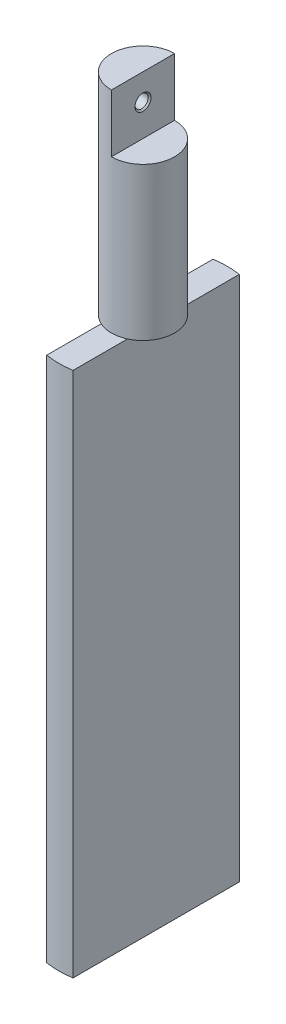
from build123d import *

# Parameters (mm, degrees)
SKETCH1_R                   = 6
BOSS_EXTRUDE1_DEPTH         = 40
CUT_EXTRUDE1_DEPTH          = 41.890096601
CUT_EXTRUDE1_DEPTH_BACK     = 41.890096601
SKETCH2_W                   = 18.470240229
SKETCH2_H                   = 11
M3_TAPPED_HOLE2_D           = 2.5
M3_TAPPED_HOLE2_CSINK_D     = 3.05
M3_TAPPED_HOLE2_CSINK_ANGLE = 90
SKETCH5_R                   = 16
BOSS_EXTRUDE2_DEPTH         = 100
CUT_EXTRUDE2_DEPTH          = 142.816783309
CUT_EXTRUDE2_DEPTH_BACK     = 100
SKETCH11_OUTSIDE_W          = 63.426
SKETCH11_OUTSIDE_H          = 63.426
SKETCH11_OUTSIDE_W_2        = 5
SKETCH11_OUTSIDE_H_2        = 40.425128238


with BuildPart() as part:
    # Sketch1 → Boss-Extrude1 (new body)
    with BuildSketch(Plane(origin=(0, 0, 0), x_dir=(1, 0, 0), z_dir=(0, 1, 0))):
        with Locations(Location((0, 0, 0), (0, 0, 270))):
            Circle(SKETCH1_R)
    extrude(amount=BOSS_EXTRUDE1_DEPTH)

    # Sketch2 → Cut-Extrude1 (cut, two sides: drawn at the far end of the back side and taken through both)
    with BuildSketch(Plane.XY.offset(-CUT_EXTRUDE1_DEPTH_BACK)):
        with Locations((9.235120115, 34.5)):
            Rectangle(SKETCH2_W, SKETCH2_H)
    extrude(amount=CUT_EXTRUDE1_DEPTH + CUT_EXTRUDE1_DEPTH_BACK, mode=Mode.SUBTRACT)

    # M3 Tapped Hole2 (through all)
    with Locations(Plane(origin=(0, 0, 0), x_dir=(0, 0, -1), z_dir=(1, 0, 0))):
        with Locations((0, 35)):
            CounterSinkHole(M3_TAPPED_HOLE2_D / 2, M3_TAPPED_HOLE2_CSINK_D / 2, counter_sink_angle=M3_TAPPED_HOLE2_CSINK_ANGLE)

    # Sketch5 → Boss-Extrude2 (add)
    with BuildSketch(Plane.XZ):
        with Locations(Location((0, 0, 0), (0, 0, 270))):
            Circle(SKETCH5_R)
    extrude(amount=BOSS_EXTRUDE2_DEPTH)

    # Sketch11 outside → Cut-Extrude2 (cut, two sides: drawn at the far end of the back side and taken through both)
    with BuildSketch(Plane.XZ.offset(100).offset(-CUT_EXTRUDE2_DEPTH_BACK)):
        Rectangle(SKETCH11_OUTSIDE_W, SKETCH11_OUTSIDE_H)
        Rectangle(SKETCH11_OUTSIDE_W_2, SKETCH11_OUTSIDE_H_2, mode=Mode.SUBTRACT)
    extrude(amount=CUT_EXTRUDE2_DEPTH + CUT_EXTRUDE2_DEPTH_BACK, mode=Mode.SUBTRACT)


solid = part.part
